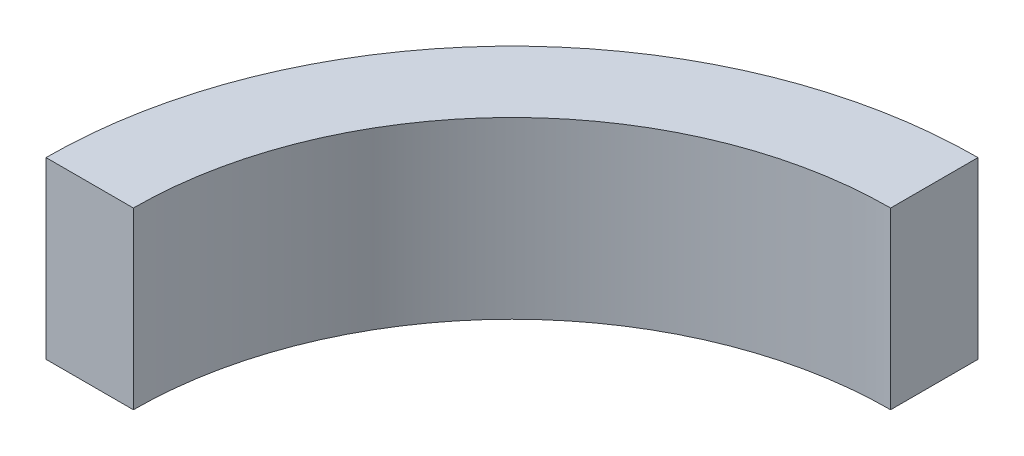
SolidWorks part; units mm, degrees
material "A3"
ref_plane "前视基准面" through (0, 0, 0) normal (0, 0, 1) x (1, 0, 0)
ref_plane "上视基准面" through (0, 0, 0) normal (0, 1, 0) x (1, 0, 0)
ref_plane "右视基准面" through (0, 0, 0) normal (1, 0, 0) x (0, 0, -1)
sketch "草图1" plane through (0, 0, 0) normal (0, 1, 0) x (1, 0, 0)
  line L0 (0, 65) -> (0, 0) construction
  line L1 (0, 0) -> (-65, 0) construction
  line L2 (-80, 0) -> (-65, 0)
  line L3 (0, 80) -> (0, 65)
  arc A0 (0, 65) -> (-65, 0) centre (0, 0) ccw
  arc A1 (0, 80) -> (-80, 0) centre (0, 0) ccw
  dimension "D1" = 130
  dimension "D2" = 15
extrude "凸台-拉伸1" add sketch "草图1" along normal blind 30
